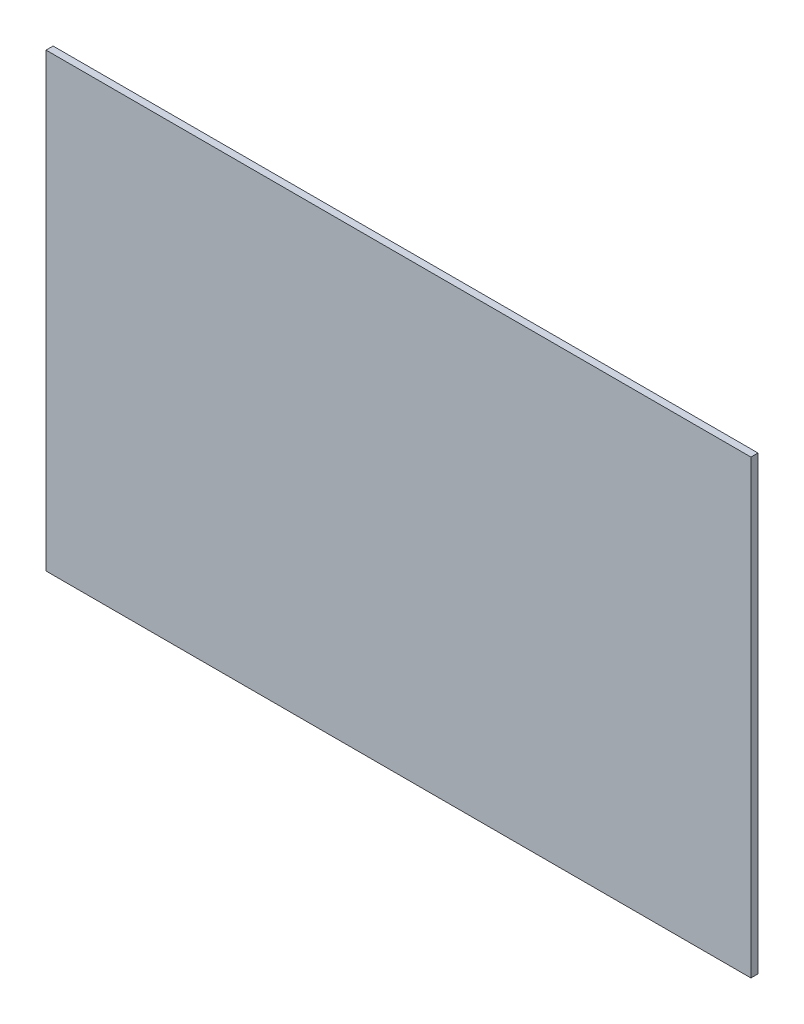
SolidWorks part; units mm, degrees
ref_plane "Front Plane" through (0, 0, 0) normal (0, 0, 1) x (1, 0, 0)
ref_plane "Top Plane" through (0, 0, 0) normal (0, 1, 0) x (1, 0, 0)
ref_plane "Right Plane" through (0, 0, 0) normal (1, 0, 0) x (0, 0, -1)
other "Configuration Table"
sketch "Sketch1" plane through (0, 0, 0) normal (0, 0, 1) x (1, 0, 0)
  line L1 (0, 0) -> (500, 0)
  line L2 (0, 0) -> (0, 320)
  line L3 (0, 320) -> (500, 320)
  line L4 (500, 0) -> (500, 320)
  dimension "D1" = 500
  dimension "D2" = 320
extrude "Boss-Extrude1" add sketch "Sketch1" along normal blind 5
